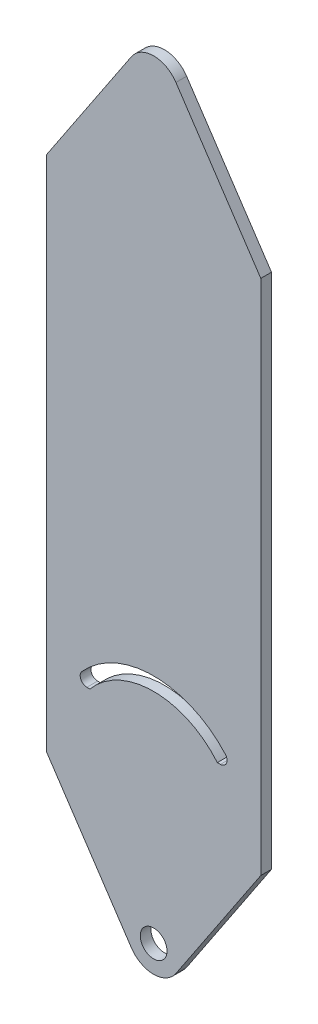
SolidWorks part; units mm, degrees
ref_plane "Front Plane" through (0, 0, 0) normal (0, 0, 1) x (1, 0, 0)
ref_plane "Top Plane" through (0, 0, 0) normal (0, 1, 0) x (1, 0, 0)
ref_plane "Right Plane" through (0, 0, 0) normal (1, 0, 0) x (0, 0, -1)
other "Configuration Table"
sketch "Sketch2" plane through (0, 0, 0) normal (0, 0, 1) x (1, 0, 0)
  line L0 (-16.6391, 618.9031) -> (-80, 713.9088)
  line L1 (-80, 713.9088) -> (-80, 1100.0912)
  line L2 (-80, 1100.0912) -> (-16.6391, 1195.0969)
  line L3 (120, 0) -> (120, 550) construction
  line L4 (0, -55) -> (0, 55) construction
  line L5 (16.6391, 618.9031) -> (80, 713.9088)
  line L6 (80, 713.9088) -> (80, 1100.0912)
  line L7 (80, 1100.0912) -> (16.6391, 1195.0969)
  circle A2 centre (0, 630) radius 10
  arc A3 (-16.6391, 618.9031) -> (16.6391, 618.9031) centre (0, 630) ccw
  arc A4 (16.6391, 1195.0969) -> (-16.6391, 1195.0969) centre (0, 1184) ccw
  circle A5 centre (0, 630) radius 10 construction
  dimension "D1" = 554
  dimension "D3" = 40
  dimension "D4" = 20
  dimension "D7" = 40
  dimension "D2" = 0
  dimension "D5" = 33.7
  dimension "D6" = 33.7
  dimension "D8" = 80
extrude "Boss-Extrude1" add sketch "Sketch2" along normal blind 8
sketch "Sketch4" plane through (0, 0, 8) normal (0, 0, 1) x (1, 0, 0)
  line L0 (-49.8493, 770.7422) -> (-47.5615, 770.7422)
  line L2 (80, 713.9088) -> (80, 1100.0912) construction
  line L3 (47.5615, 770.7422) -> (49.8493, 770.7422)
  arc A0 (-53.5752, 779.0765) -> (53.5752, 779.0765) centre (0, 731.1325) cw
  arc A1 (-47.5615, 770.7422) -> (47.5615, 770.7422) centre (0, 731.1325) cw
  arc A2 (-51.6545, 765.2328) -> (51.6545, 765.2328) centre (0, 731.1325) cw construction
  arc A3 (-60, 770.7422) -> (60, 770.7422) centre (0, 731.1325) cw construction
  arc A4 (49.8493, 770.7422) -> (53.5752, 779.0765) centre (49.8493, 775.7422) ccw
  arc A5 (-49.8493, 770.7422) -> (-53.5752, 779.0765) centre (-49.8493, 775.7422) cw
  point P15 (60, 770.7422)
  dimension "D4" = 5
  dimension "D1" = 20
  dimension "D3" = 10
extrude "Cut-Extrude1" cut sketch "Sketch4" against normal blind 10
